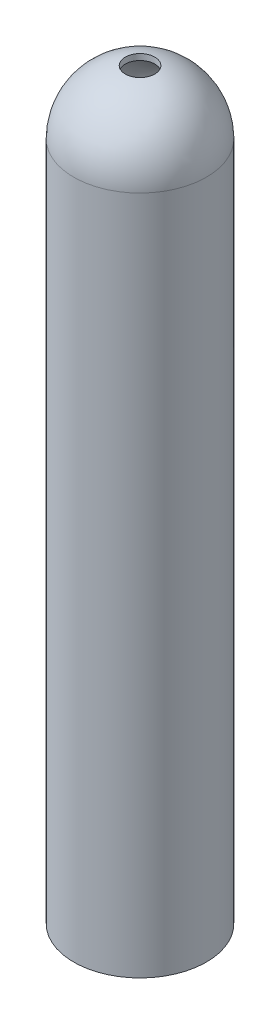
SolidWorks part; units mm, degrees
material "铜"
ref_plane "Front Plane" through (0, 0, 0) normal (0, 0, 1) x (1, 0, 0)
ref_plane "Top Plane" through (0, 0, 0) normal (0, 1, 0) x (1, 0, 0)
ref_plane "Right Plane" through (0, 0, 0) normal (1, 0, 0) x (0, 0, -1)
sketch "Sketch1" plane through (0, 0, 0) normal (0, 0, 1) x (1, 0, 0)
  line L0 (-2.25, 0) -> (-2.25, 23.0465)
  line L1 (-2.05, 0) -> (-2.05, 23.0465)
  line L3 (0, 0) -> (0, 27.9134) construction
  line L4 (-2.25, 0) -> (-2.05, 0)
  line L5 (-0.5, 25.2) -> (-0.5, 24.9952)
  arc A0 (-2.25, 23.0465) -> (-0.5, 25.2) centre (-0.05, 23.0465) cw
  arc A1 (-2.05, 23.0465) -> (-0.5, 24.9952) centre (-0.05, 23.0465) cw
  arc A3 (-2.05, 23.0465) -> (-0.05, 25.0465) centre (-0.05, 23.0465) cw construction
  arc A4 (-2.25, 23.0465) -> (-0.05, 25.2465) centre (-0.05, 23.0465) cw construction
  dimension "D1" = 0.2
  dimension "D2" = 4.5
  dimension "D3" = 25.2
  dimension "D4" = 1
revolve "Revolve1" add sketch "Sketch1" angle 360 about L3
